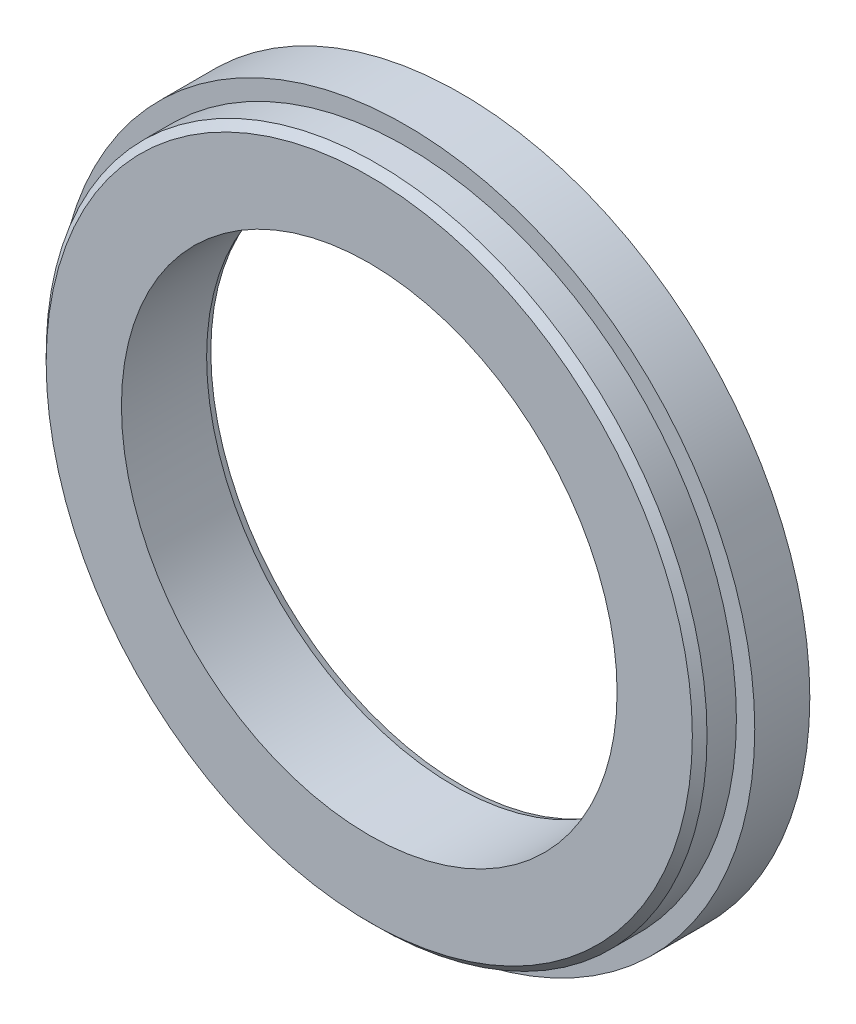
SolidWorks part; units mm, degrees
ref_plane "Front Plane" through (0, 0, 0) normal (0, 0, 1) x (1, 0, 0)
ref_plane "Top Plane" through (0, 0, 0) normal (0, 1, 0) x (1, 0, 0)
ref_plane "Right Plane" through (0, 0, 0) normal (1, 0, 0) x (0, 0, -1)
sketch "Sketch1" plane through (0, 0, 0) normal (0, 0, 1) x (1, 0, 0)
  circle A0 centre (0, 0) radius 95
  circle A1 centre (0, 0) radius 67.5
extrude "Boss-Extrude1" add sketch "Sketch1" along normal blind 15
sketch "Sketch2" plane through (0, 0, 15) normal (0, 0, 1) x (1, 0, 0)
  circle A0 centre (0, 0) radius 90
  circle A1 centre (0, 0) radius 67.5
extrude "Boss-Extrude2" add sketch "Sketch2" along normal blind 10
chamfer "Chamfer1" distance 2 angle 45 1 edges at (90, 0, 25)
chamfer "Chamfer2" distance 1.8 angle 20 1 edges at (67.5, 0, 0)
sketch "Sketch3" plane through (0, 0, 0) normal (0, 0, -1) x (-1, 0, 0)
  circle A0 centre (80.5, 0) radius 5.75
  circle A1 centre (40.25, -69.715) radius 5.75
  circle A2 centre (-40.25, -69.715) radius 5.75
  circle A3 centre (-80.5, 0) radius 5.75
  circle A4 centre (-40.25, 69.715) radius 5.75
  circle A5 centre (40.25, 69.715) radius 5.75
  point P17 (0, 0)
  dimension "D1" = 6
hole_wizard "M12x1.5 Tapped Hole1" positions "3DSketch1" profile "Sketch4" tap size "M12x1.5" standard "Ansi Metric"
sketch3d "3DSketch1"
  point P0 (40.25, 69.715, 0)
  point P3 (-40.25, 69.715, 0)
  point P6 (-80.5, 0, 0)
  point P9 (-40.25, -69.715, 0)
  point P13 (80.5, 0, 0)
  point P16 (40.25, -69.715, 0)
sketch "Sketch4" plane through (40.25, 69.715, 0) normal (1, 0, 0) x (0, 1, 0)
  line L0 (0, 0) -> (0, 23.1545)
  line L1 (0, 23.1545) -> (5.25, 20)
  line L2 (5.25, 20) -> (5.25, 0)
  line L5 (5.25, 0) -> (0, 0)
  line L10 (0, 23.1545) -> (-5.25, 20) construction
  line L11 (0, -6.35) -> (0, 107.95) construction
  dimension "螺纹孔钻头直径" = 10.5
  dimension "螺纹孔钻头深度" = 20
  dimension "导头角度" = 118
cosmetic thread "Hole Thread Line1" parameters "D1"=15, "D2"=12
cosmetic thread "Hole Thread Line2" parameters "D1"=15, "D2"=12
cosmetic thread "Hole Thread Line3" parameters "D1"=15, "D2"=12
cosmetic thread "Hole Thread Line4" parameters "D1"=15, "D2"=12
cosmetic thread "Hole Thread Line5" parameters "D1"=15, "D2"=12
cosmetic thread "Hole Thread Line6" parameters "D1"=15, "D2"=12
